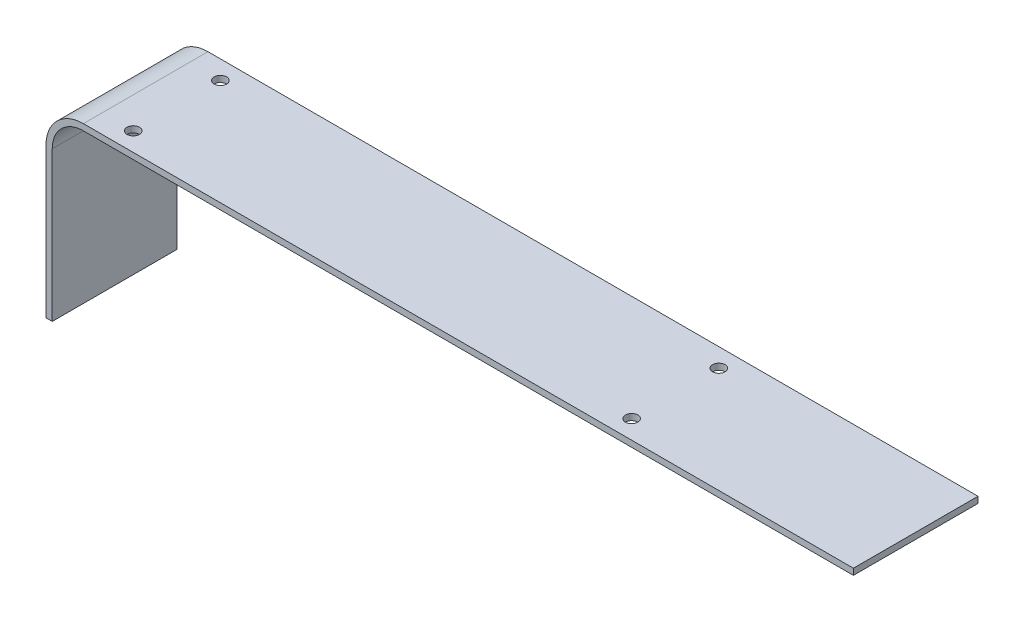
SolidWorks part; units mm, degrees
material "Plain Carbon Steel"
ref_plane "Front Plane" through (0, 0, 0) normal (0, 0, 1) x (1, 0, 0)
ref_plane "Top Plane" through (0, 0, 0) normal (0, 1, 0) x (1, 0, 0)
ref_plane "Right Plane" through (0, 0, 0) normal (1, 0, 0) x (0, 0, -1)
sketch "Sketch1" plane through (0, 0, 0) normal (0, 0, 1) x (1, 0, 0)
  line L0 (0, 0) -> (0, 120)
  line L1 (30, 150) -> (648, 150)
  arc A0 (30, 150) -> (0, 120) centre (30, 120) ccw
  point P6 (0, 150)
  dimension "D3" = 30
  dimension "D1" = 150
  dimension "D2" = 648
extrude "Extrude-Thin1" add sketch "Sketch1" along normal blind 100 thin
sketch "Sketch2" plane through (0, 145, 0) normal (0, -1, 0) x (1, 0, 0)
  line L0 (0, 100) -> (0, 0) construction
  line L1 (30, 100) -> (648, 100) construction
  circle A0 centre (55, 85) radius 5
  dimension "D2" = 10
  dimension "D1" = 55
  dimension "D3" = 15
extrude "Cut-Extrude1" cut sketch "Sketch2" against normal blind 10
pattern_linear "LPattern1" count 2 spacing 400 along (1, 0, 0) count 2 spacing 70 along (0, 0, -1) of "Cut-Extrude1"
